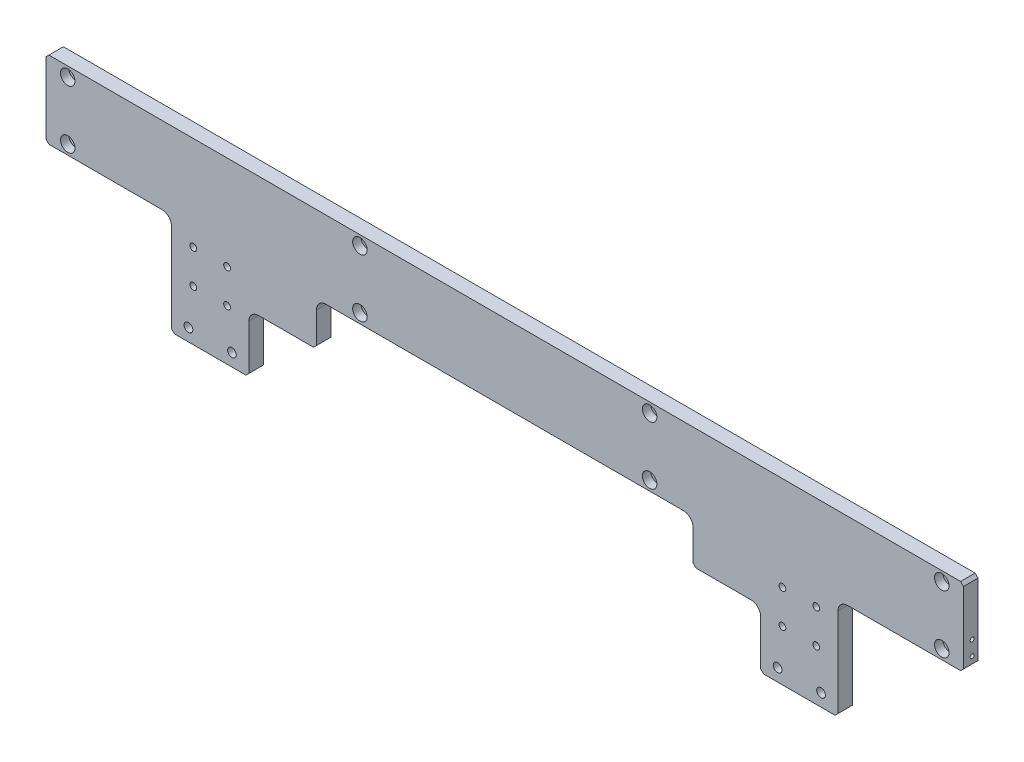
from build123d import *

# Parameters (mm, degrees)
SKETCH_1_W                   = 950
SKETCH_1_H                   = 80
EXTRUDE_1_DEPTH              = 7.5
HOLE_WIZARD_M8_1_D           = 9
HOLE_WIZARD_M8_1_CBORE_D     = 15
HOLE_WIZARD_M8_1_CBORE_DEPTH = 8.6
CHAMFER_1_SIZE               = 3
SKETCH_7_W                   = 150
SKETCH_7_H                   = 15
EXTRUDE_2_DEPTH              = 105
FILLET_1_R                   = 10
HOLE_WIZARD_M6_1_D           = 7
HOLE_WIZARD_9_0_9_1_D        = 9
HOLE_WIZARD_M5_1_D           = 4.2
HOLE_WIZARD_M5_1_DEPTH       = 12.4
HOLE_WIZARD_M5_1_TIP         = 1.2618073
HOLE_WIZARD_M5_2_D           = 4.2
HOLE_WIZARD_M5_2_DEPTH       = 12.4
HOLE_WIZARD_M5_2_TIP         = 1.2618073
SKETCH_17_W                  = 70
SKETCH_17_H                  = 60
CUT_EXTRUDE_1_DEPTH          = 497.865172859
FILLET_2_R                   = 10
CHAMFER_3_SIZE               = 3


with BuildPart() as part:
    # 草图1 → 凸台-拉伸1 (new, symmetric)
    with BuildSketch(Plane.XY):
        Rectangle(SKETCH_1_W, SKETCH_1_H)
    extrude(amount=EXTRUDE_1_DEPTH, both=True)

    # M8 六角凹头螺钉的柱形沉头孔1 (through all)
    with Locations(Plane.XY.offset(7.5)):
        with Locations((452.5, -30), (452.5, 30), (150, -30), (150, 30), (-452.5, 30), (-452.5, -30), (-150, 30), (-150, -30)):
            CounterBoreHole(HOLE_WIZARD_M8_1_D / 2, HOLE_WIZARD_M8_1_CBORE_D / 2, HOLE_WIZARD_M8_1_CBORE_DEPTH)

    # 倒角1
    chamfer_1_edges = [part.edges().sort_by_distance(p)[0] for p in [
        (475, -40, 0),
        (-475, -40, 0),
        (-475, 40, 0),
        (475, 40, 0),
    ]]
    chamfer(chamfer_1_edges, length=CHAMFER_1_SIZE)

    # 草图7 → 凸台-拉伸2 (add)
    with BuildSketch(Plane.XZ.offset(40)):
        with Locations((270, 0)):
            Rectangle(SKETCH_7_W, SKETCH_7_H)
    extrude_2 = extrude(amount=EXTRUDE_2_DEPTH)

    # 镜向1: 凸台-拉伸2 across plane
    add(extrude_2.mirror(Plane(origin=(0, 0, 0), x_dir=(0, 0, 1), z_dir=(1, 0, 0))))

    # 圆角1
    fillet_1_edges = [part.edges().sort_by_distance(p)[0] for p in [
        (-345, -40, 0),
        (-195, -40, 0),
        (195, -40, 0),
        (345, -40, 0),
    ]]
    fillet(fillet_1_edges, radius=FILLET_1_R)

    # M6 六角凹头螺钉的柱形沉头孔1 (through all)
    with Locations(Plane(origin=(0, 0, -7.5), x_dir=(-1, 0, 0), z_dir=(0, 0, -1))):
        with Locations((-287.5, -92.5), (-287.5, -57.5), (-322.5, -57.5), (-322.5, -92.5)):
            hole_wizard_m6_1 = Hole(HOLE_WIZARD_M6_1_D / 2)

    # Ø9.0 (9) 直径孔1 (through all)
    with Locations(Plane(origin=(0, 0, -7.5), x_dir=(-1, 0, 0), z_dir=(0, 0, -1))):
        with Locations((-282.5, -132), (-327.5, -132)):
            hole_wizard_9_0_9_1 = Hole(HOLE_WIZARD_9_0_9_1_D / 2)

    # 镜向2: M6 六角凹头螺钉的柱形沉头孔1, Ø9.0 (9) 直径孔1 across plane
    add(hole_wizard_m6_1.mirror(Plane(origin=(0, 0, 0), x_dir=(0, 0, 1), z_dir=(1, 0, 0))), mode=Mode.SUBTRACT)
    add(hole_wizard_9_0_9_1.mirror(Plane(origin=(0, 0, 0), x_dir=(0, 0, 1), z_dir=(1, 0, 0))), mode=Mode.SUBTRACT)

    # M5 螺纹孔1
    with Locations(Plane.ZY.offset(475)):
        with Locations((-1.5, -30), (-1.5, -15)):
            Hole(HOLE_WIZARD_M5_1_D / 2, depth=HOLE_WIZARD_M5_1_DEPTH)
            with Locations((0, 0, -(HOLE_WIZARD_M5_1_DEPTH + HOLE_WIZARD_M5_1_TIP / 2))):  # 118° drill point
                Cone(0, HOLE_WIZARD_M5_1_D / 2, HOLE_WIZARD_M5_1_TIP, mode=Mode.SUBTRACT)

    # M5 螺纹孔2
    with Locations(Plane(origin=(475, 0, 0), x_dir=(0, 0, -1), z_dir=(1, 0, 0))):
        with Locations((1.5, -15), (1.5, -30)):
            Hole(HOLE_WIZARD_M5_2_D / 2, depth=HOLE_WIZARD_M5_2_DEPTH)
            with Locations((0, 0, -(HOLE_WIZARD_M5_2_DEPTH + HOLE_WIZARD_M5_2_TIP / 2))):  # 118° drill point
                Cone(0, HOLE_WIZARD_M5_2_D / 2, HOLE_WIZARD_M5_2_TIP, mode=Mode.SUBTRACT)

    # 草图17 → 切除-拉伸1 (cut, through all)
    with BuildSketch(Plane(origin=(0, 0, -7.5), x_dir=(-1, 0, 0), z_dir=(0, 0, -1))):
        with Locations((-230, -115)):
            Rectangle(SKETCH_17_W, SKETCH_17_H)
    cut_extrude_1 = extrude(amount=-CUT_EXTRUDE_1_DEPTH, mode=Mode.SUBTRACT)

    # 镜向3: 切除-拉伸1 across plane
    add(cut_extrude_1.mirror(Plane(origin=(0, 0, 0), x_dir=(0, 0, 1), z_dir=(1, 0, 0))), mode=Mode.SUBTRACT)

    # 圆角2
    fillet_2_edges = [part.edges().sort_by_distance(p)[0] for p in [
        (265, -85, 0),
        (-265, -85, 0),
    ]]
    fillet(fillet_2_edges, radius=FILLET_2_R)

    # 倒角3
    chamfer_3_edges = [part.edges().sort_by_distance(p)[0] for p in [
        (-345, -145, 0),
        (-265, -145, 0),
        (-195, -85, 0),
        (195, -85, 0),
        (265, -145, 0),
        (345, -145, 0),
    ]]
    chamfer(chamfer_3_edges, length=CHAMFER_3_SIZE)


solid = part.part
